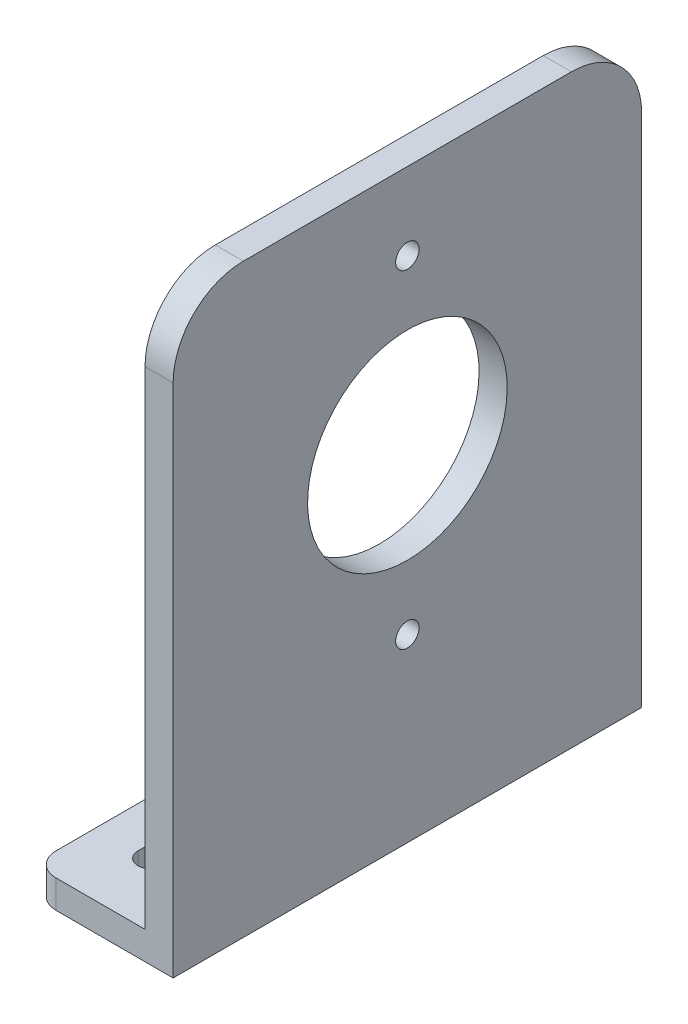
SolidWorks part; units mm, degrees
ref_plane "Front Plane" through (0, 0, 0) normal (0, 0, 1) x (1, 0, 0)
ref_plane "Top Plane" through (0, 0, 0) normal (0, 1, 0) x (1, 0, 0)
ref_plane "Right Plane" through (0, 0, 0) normal (1, 0, 0) x (0, 0, -1)
sketch "Sketch 1" plane through (0, 0, 0) normal (0, 0, 1) x (1, 0, 0)
  line L0 (0, 297.8334) -> (0, -63.6364) construction
  line L1 (-94.5455, 0) -> (56.3636, 0) construction
  line L2 (-60, 0) -> (0, 0)
  line L3 (0, 0) -> (0, 250)
  line L4 (0, 250) -> (-12, 250)
  line L5 (-12, 250) -> (-12, 12)
  line L6 (-12, 12) -> (-60, 12)
  line L7 (-60, 12) -> (-60, 0)
  dimension "D1" = 60
  dimension "D2" = 250
  dimension "D3" = 12
  dimension "D4" = 12
extrude "Boss-Extrude 1" add sketch "Sketch 1" along normal mid plane 200
sketch "Sketch 2" plane through (0, 12, 0) normal (0, 1, 0) x (1, 0, 0)
  line L0 (-73.662, 0) -> (21.6388, 0) construction
  line L1 (-37, 67.5) -> (-37, 72.5) construction
  line L2 (-42.5, 67.5) -> (-42.5, 72.5)
  line L3 (-31.5, 67.5) -> (-31.5, 72.5)
  line L4 (0, -100) -> (0, 100) construction
  line L5 (-37, -67.5) -> (-37, -72.5) construction
  line L6 (-42.5, -67.5) -> (-42.5, -72.5)
  line L7 (-31.5, -67.5) -> (-31.5, -72.5)
  arc A0 (-42.5, 67.5) -> (-31.5, 67.5) centre (-37, 67.5) ccw
  arc A1 (-31.5, 72.5) -> (-42.5, 72.5) centre (-37, 72.5) ccw
  arc A2 (-42.5, -67.5) -> (-31.5, -67.5) centre (-37, -67.5) cw
  arc A3 (-31.5, -72.5) -> (-42.5, -72.5) centre (-37, -72.5) cw
  point P5 (-37, 70)
  point P14 (-37, -70)
  dimension "D1" = 140
  dimension "D2" = 11
  dimension "D3" = 5
  dimension "D4" = 37
extrude "Cut-Extrude 1" cut sketch "Sketch 2" against normal through all
sketch "Sketch 3" plane through (-12, 0, 0) normal (-1, 0, 0) x (0, 0, 1)
  line L0 (0, 307.8222) -> (0, -29.5174) construction
  line L1 (100, 0) -> (-100, 0) construction
  line L2 (-82.1061, 147) -> (112.6469, 147) construction
  circle A0 centre (0, 147) radius 42.6
  circle A1 centre (0, 217) radius 5
  circle A2 centre (0, 77) radius 5
  dimension "D1" = 85.2
  dimension "D2" = 147
  dimension "D3" = 10
  dimension "D4" = 140
extrude "Cut-Extrude 2" cut sketch "Sketch 3" against normal through all
fillet "Fillet 1" radius 30 2 edges at (-6, 250, -100) (-6, 250, 100)
fillet "Fillet 2" radius 10 2 edges at (-60, 6, -100) (-60, 6, 100)
